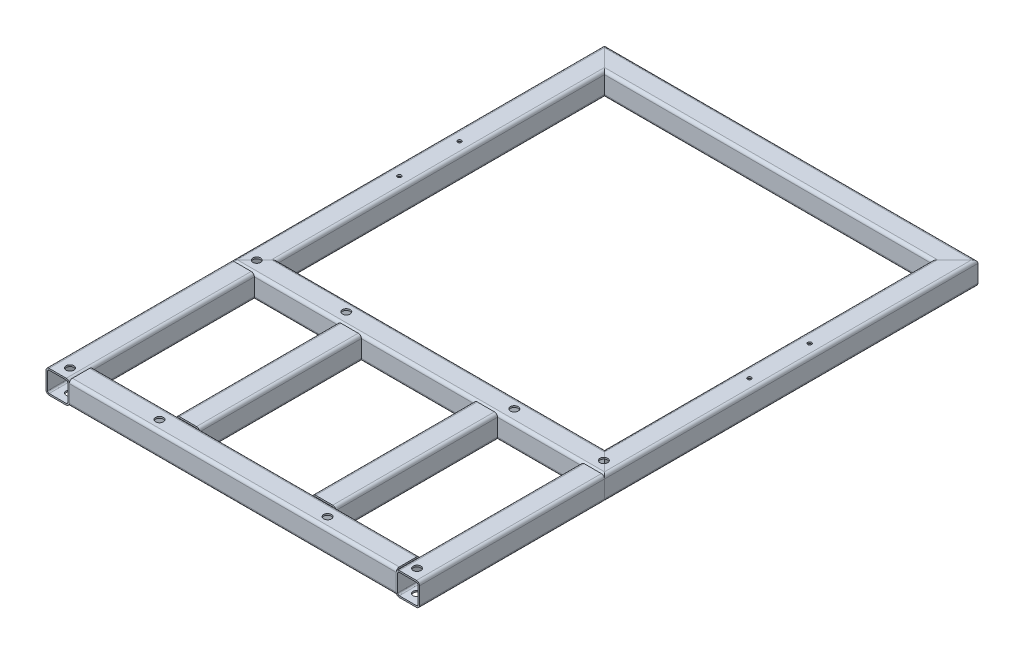
SolidWorks part; units mm, degrees
ref_plane "前视基准面" through (0, 0, 0) normal (0, 0, 1) x (1, 0, 0)
ref_plane "上视基准面" through (0, 0, 0) normal (0, 1, 0) x (1, 0, 0)
ref_plane "右视基准面" through (0, 0, 0) normal (1, 0, 0) x (0, 0, -1)
sketch "草图1" plane through (0, 0, 0) normal (0, 1, 0) x (1, 0, 0)
  line L0 (-450, -450) -> (-450, -925.5)
  line L1 (-450, -450) -> (450, -450)
  line L2 (-450, -450) -> (-450, 450)
  line L3 (-450, 450) -> (450, 450)
  line L4 (450, -450) -> (450, 450)
  line L5 (-450, -450) -> (450, 450) construction
  line L6 (-450, 450) -> (450, -450) construction
  line L7 (-450, -925.5) -> (450, -925.5)
  line L8 (450, -925.5) -> (450, -450)
  line L9 (-175, -450) -> (-175, -925.5)
  line L10 (175, -450) -> (175, -925.5)
  line L11 (0, 975.1164) -> (0, -1823.8011) construction
  point P0 (0, 0)
  dimension "D1" = 900
  dimension "D2" = 900
  dimension "D3" = 350
  dimension "D4" = 475.5
other "Gb／6728-1986方形空心型钢 060 X 60 X 4(1)"
ref_plane "基准面1" through (-450, 0, 450) normal (0, 0, -1) x (-1, 0, 0)
sketch "Sketch127" plane through (-450, 0, 450) normal (0, 0, -1) x (-1, 0, 0)
  line L0 (-22, -26) -> (22, -26)
  line L1 (-26, -22) -> (-26, 22)
  line L2 (22, 26) -> (-22, 26)
  line L3 (26, 22) -> (26, -22)
  line L4 (-22, -30) -> (22, -30)
  line L5 (-30, -22) -> (-30, 22)
  line L6 (22, 30) -> (-22, 30)
  line L7 (30, 22) -> (30, -22)
  arc A0 (30, 22) -> (22, 30) centre (22, 22) ccw
  arc A1 (22, -30) -> (30, -22) centre (22, -22) ccw
  arc A2 (-30, -22) -> (-22, -30) centre (-22, -22) ccw
  arc A3 (-22, 30) -> (-30, 22) centre (-22, 22) ccw
  arc A4 (-22, 26) -> (-26, 22) centre (-22, 22) ccw
  arc A5 (26, 22) -> (22, 26) centre (22, 22) ccw
  arc A6 (22, -26) -> (26, -22) centre (22, -22) ccw
  arc A7 (-26, -22) -> (-22, -26) centre (-22, -22) ccw
  point P0 (-30, 0)
  point P1 (30, 0)
  point P2 (0, 30)
  point P3 (0, -30)
  point P4 (0, 0)
  point P5 (-30, -30)
  point P6 (30, -30)
  point P7 (30, 30)
  point P8 (-30, 30)
  point P33 (0, 0)
  dimension "D1" = 8
  dimension "Thickness" = 4
  dimension "V_leg" = 60
sketch "草图2" plane through (0, 30, 0) normal (0, 1, 0) x (1, 0, 0)
  line L0 (420, 420) -> (480, 420) construction
  line L1 (480, -480) -> (480, 480) construction
  line L2 (450, 420) -> (450, -480) construction
  line L3 (-480, -480) -> (480, -480) construction
  line L5 (0, 0) -> (0, 231.7192) construction
  line L6 (0, 0) -> (-659.0776, 0) construction
  circle A0 centre (450, 77.5) radius 5
  circle A1 centre (450, -77.5) radius 5
  circle A2 centre (-450, -77.5) radius 5
  circle A3 centre (-450, 77.5) radius 5
  dimension "D1" = 10
  dimension "D2" = 10
  dimension "D3" = 155
  dimension "D4" = 77.5
extrude "切除-拉伸1" cut sketch "草图2" against normal blind 90
sketch "草图3" plane through (0, 0, 0) normal (0, 1, 0) x (1, 0, 0)
  line L0 (-420, 0) -> (420, 0)
  line L1 (-420, 420) -> (-420, -420) construction
  line L2 (420, -420) -> (420, 420) construction
ref_plane "基准面3" through (0, -150, 0) normal (0, 1, 0) x (1, 0, 0)
sketch "草图6" plane through (0, 0, 0) normal (0, 1, 0) x (1, 0, 0)
  line L0 (-322.39, 480) -> (-322.39, 780)
  line L2 (-420, 420) -> (-420, -420) construction
  line L3 (-22.39, 480) -> (-22.39, 780)
  line L4 (277.61, 480) -> (277.61, 780)
  line L5 (480, 480) -> (-480, 480) construction
  dimension "D1" = 97.61
  dimension "D3" = 300
  dimension "D2" = 3
sketch "草图7" plane through (0, 30, 0) normal (0, 1, 0) x (1, 0, 0)
  line L0 (472, -955.5) -> (428, -955.5) construction
  line L1 (480, -955.5) -> (480, -480) construction
  circle A0 centre (446, -927.75) radius 10
  dimension "D1" = 20
  dimension "D3" = 34
  dimension "D2" = 27.75
extrude "切除-拉伸2" cut sketch "草图7" against normal blind 400
ref_plane "基准面5" through (-322.39, 0, 0) normal (1, 0, 0) x (0, 0, -1)
ref_plane "基准面6" through (277.61, 0, 0) normal (1, 0, 0) x (0, 0, -1)
pattern_linear "阵列(线性)1" count 2 spacing 230 along (-1, 0, 0) of "切除-拉伸2"
mirror "镜向3" about plane through (0, 0, 0) normal (1, 0, 0) of "阵列(线性)1", "切除-拉伸2"
ref_plane "基准面7" through (0, 0, 687.75) normal (0, 0, 1) x (1, 0, 0)
mirror "镜向4" about plane through (0, 0, 687.75) normal (0, 0, 1) of "镜向3", "阵列(线性)1", "切除-拉伸2"
